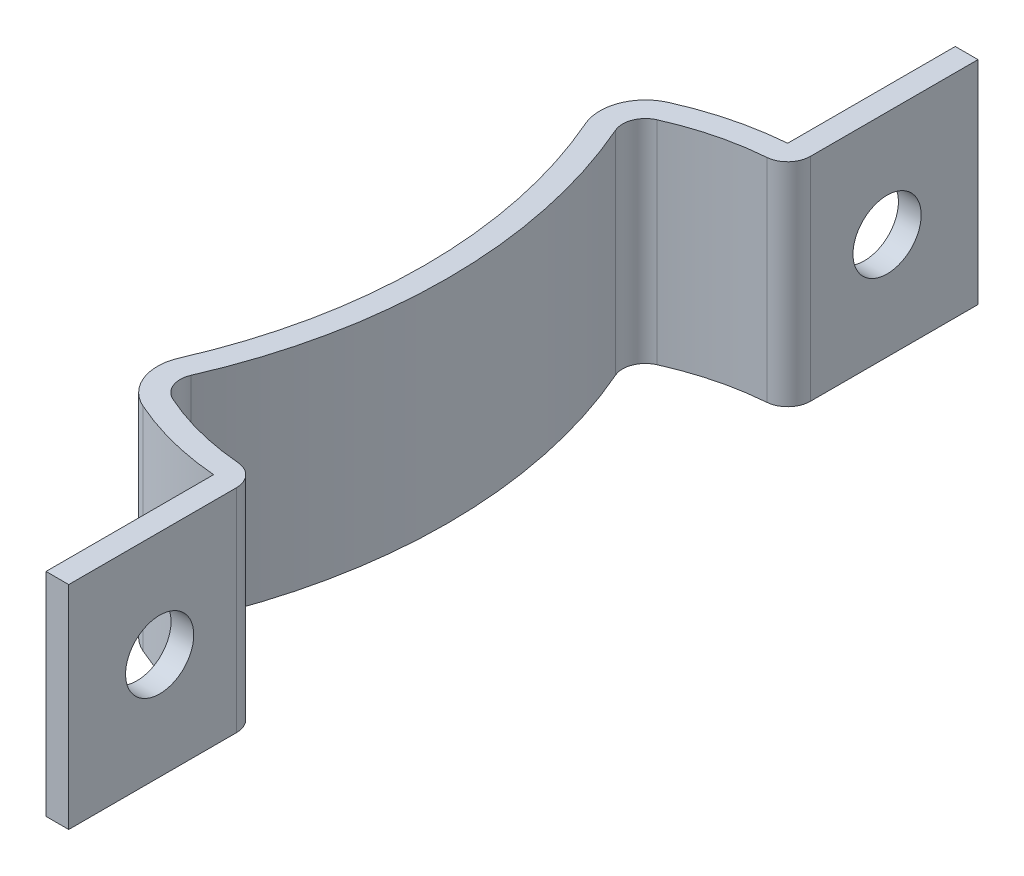
SolidWorks part; units mm, degrees
ref_plane "Front Plane" through (0, 0, 0) normal (0, 0, 1) x (1, 0, 0)
ref_plane "Top Plane" through (0, 0, 0) normal (0, 1, 0) x (1, 0, 0)
ref_plane "Right Plane" through (0, 0, 0) normal (1, 0, 0) x (0, 0, -1)
sketch "Sketch1" plane through (0, 0, 0) normal (0, 1, 0) x (1, 0, 0)
  line L0 (0, 18.9407) -> (0, 30)
  line L1 (0, -18.9407) -> (0, -30)
  arc A0 (-7.9217, -13.9993) -> (-7.9217, 13.9993) centre (-40, 0) ccw
  arc A1 (-1.3816, 17.4454) -> (-7.1606, 15.9679) centre (0, 0) ccw
  arc A2 (-7.1606, -15.9679) -> (-1.3816, -17.4454) centre (0, 0) ccw
  arc A3 (0, 18.9407) -> (-1.3816, 17.4454) centre (-1.5, 18.9407) cw
  arc A4 (0, -18.9407) -> (-1.3816, -17.4454) centre (-1.5, -18.9407) ccw
  arc A5 (-7.1606, -15.9679) -> (-7.9217, -13.9993) centre (-6.5469, -14.5993) cw
  arc A6 (-7.9217, 13.9993) -> (-7.1606, 15.9679) centre (-6.5469, 14.5993) cw
  point P10 (0, 17.5)
  point P13 (0, -17.5)
  point P16 (-8.5156, -15.2884)
  dimension "D1" = 70
  dimension "D4" = 12.5
  dimension "D5" = 12.5
  dimension "D6" = 1.5
  dimension "D3" = 35
  dimension "D2" = 40
extrude "Extrude-Thin3" add sketch "Sketch1" along normal blind 14 thin
sketch "Sketch3" plane through (0, 0, 0) normal (1, 0, 0) x (0, 0, -1)
  line L0 (30, 7) -> (-30, 7) construction
  line L1 (30, 14) -> (30, 0) construction
  line L2 (-30, 14) -> (-30, 0) construction
  circle A0 centre (-24, 7) radius 2.25
  circle A1 centre (24, 7) radius 2.25
  dimension "D1" = 4.5
  dimension "D2" = 4.5
  dimension "D3" = 48
  dimension "D4" = 24
extrude "Cut-Extrude2" cut sketch "Sketch3" against normal up to next
